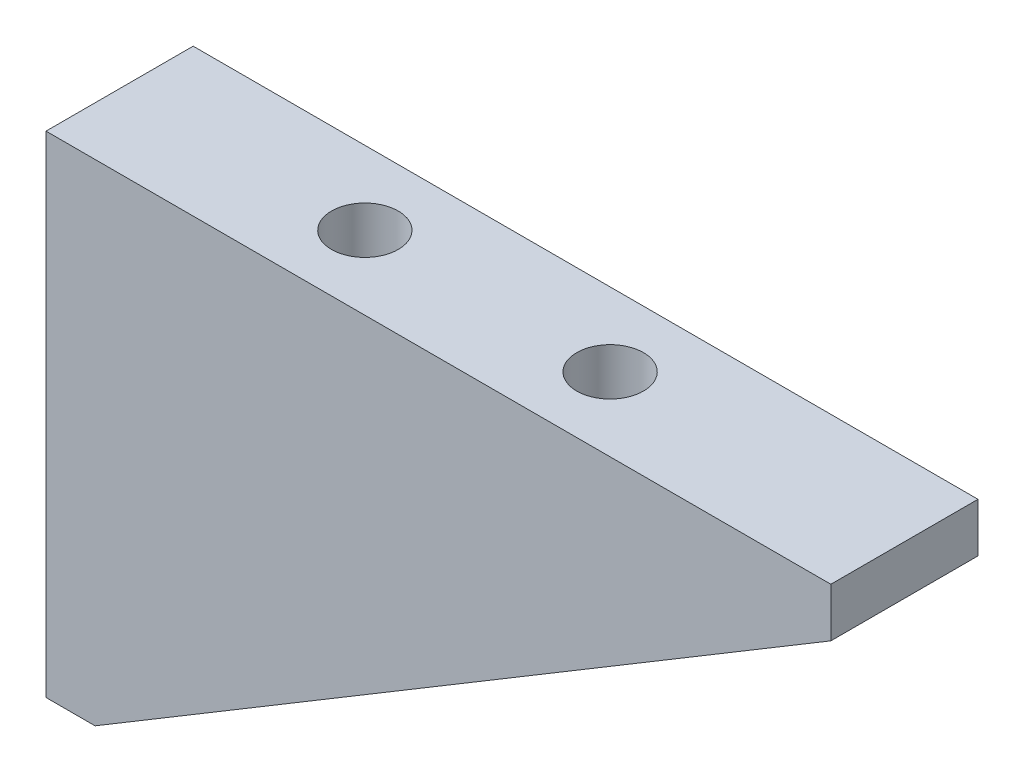
from build123d import *

# Parameters (mm, degrees)
BOSS_EXTRUDE1_DEPTH   = 15
M8_TAPPED_HOLE1_D     = 6.8
M8_TAPPED_HOLE1_DEPTH = 22.25
M8_TAPPED_HOLE1_TIP   = 2.042926105
M8_TAPPED_HOLE2_D     = 6.8
M8_TAPPED_HOLE2_DEPTH = 22.25
M8_TAPPED_HOLE2_TIP   = 2.042926105


with BuildPart() as part:
    # Sketch1 → Boss-Extrude1 (new body)
    with BuildSketch(Plane.XY):
        Polygon((0, 0), (0, 50), (80, 50), (80, 45), (5, 0), align=None)
    extrude(amount=BOSS_EXTRUDE1_DEPTH)

    # M8 Tapped Hole1
    with Locations(Plane(origin=(0, 50, 0), x_dir=(1, 0, 0), z_dir=(0, 1, 0))):
        with Locations((25, -7.5), (50, -7.5)):
            Hole(M8_TAPPED_HOLE1_D / 2, depth=M8_TAPPED_HOLE1_DEPTH)
            with Locations((0, 0, -(M8_TAPPED_HOLE1_DEPTH + M8_TAPPED_HOLE1_TIP / 2))):  # 118° drill point
                Cone(0, M8_TAPPED_HOLE1_D / 2, M8_TAPPED_HOLE1_TIP, mode=Mode.SUBTRACT)

    # M8 Tapped Hole2
    with Locations(Plane.ZY):
        with Locations((7.5, 35), (7.5, 15)):
            Hole(M8_TAPPED_HOLE2_D / 2, depth=M8_TAPPED_HOLE2_DEPTH)
            with Locations((0, 0, -(M8_TAPPED_HOLE2_DEPTH + M8_TAPPED_HOLE2_TIP / 2))):  # 118° drill point
                Cone(0, M8_TAPPED_HOLE2_D / 2, M8_TAPPED_HOLE2_TIP, mode=Mode.SUBTRACT)


solid = part.part
